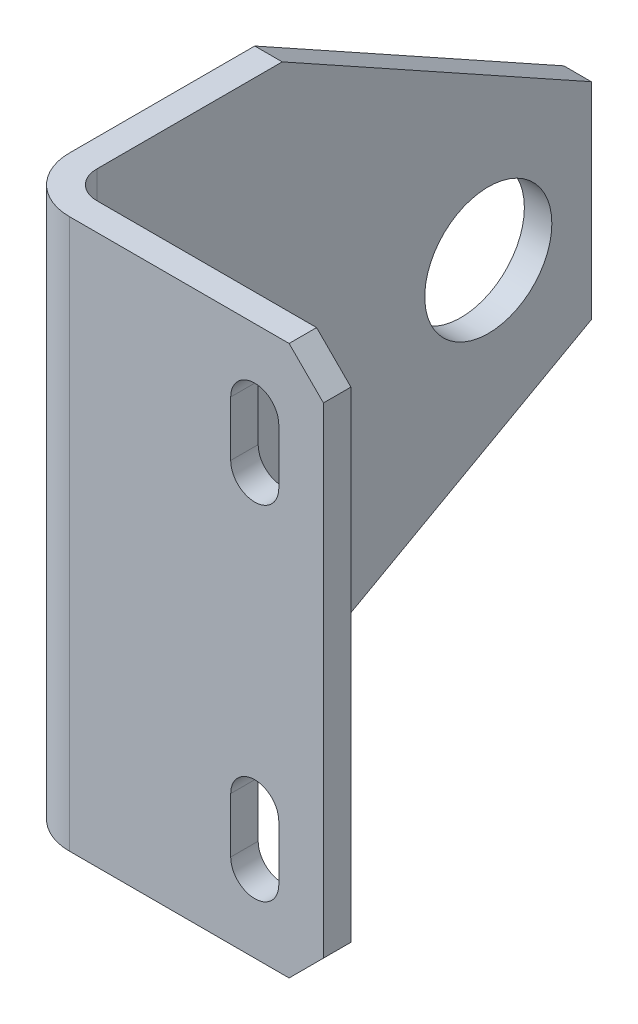
from build123d import *

# Parameters (mm, degrees)
EXTRUDE_1_DEPTH           = 4
SKETCH_2_W                = 4
SKETCH_2_H                = 80
EXTRUDE_2_DEPTH           = 41
CUT_EXTRUDE_1_DEPTH       = 140.749776386
CUT_EXTRUDE_2_DEPTH       = 137.711374801
HOLE_WIZARD_18_5_18_5_1_D = 18.5
CHAMFER_1_SIZE            = 5
CHAMFER_2_SIZE            = 30.886890423
FILLET_1_R                = 4
FILLET_2_R                = 8


with BuildPart() as part:
    # 草图1 → 凸台-拉伸1 (new body)
    with BuildSketch(Plane(origin=(0, 0, 0), x_dir=(0, 0, -1), z_dir=(1, 0, 0))):
        Polygon((-45, 0), (27, 40), (-45, 80), (-80, 80), (-80, 0), align=None)
    extrude(amount=-EXTRUDE_1_DEPTH)

    # 草图2 → 凸台-拉伸2 (add)
    with BuildSketch(Plane(origin=(0, 0, 0), x_dir=(0, 0, -1), z_dir=(1, 0, 0))):
        with Locations((-78, 40)):
            Rectangle(SKETCH_2_W, SKETCH_2_H)
    extrude(amount=EXTRUDE_2_DEPTH)

    # 草图3 → 切除-拉伸1 (cut, through all)
    with BuildSketch(Plane.XY.offset(80)):
        with BuildLine():
            Line((34.5, 61), (34.5, 69))
            ThreePointArc((34.5, 69), (31, 72.5), (27.5, 69))
            Line((27.5, 69), (27.5, 61))
            ThreePointArc((27.5, 61), (31, 57.5), (34.5, 61))
        make_face()
    extrude(amount=-CUT_EXTRUDE_1_DEPTH, mode=Mode.SUBTRACT)

    # 草图4 → 切除-拉伸2 (cut, through all)
    with BuildSketch(Plane(origin=(0, 0, 76), x_dir=(-1, 0, 0), z_dir=(0, 0, -1))):
        with BuildLine():
            Line((-34.5, 19), (-34.5, 11))
            ThreePointArc((-34.5, 11), (-31, 7.5), (-27.5, 11))
            Line((-27.5, 11), (-27.5, 19))
            ThreePointArc((-27.5, 19), (-31, 22.5), (-34.5, 19))
        make_face()
    extrude(amount=-CUT_EXTRUDE_2_DEPTH, mode=Mode.SUBTRACT)

    # Ø18.5 (18.5) 直径孔1 (through all)
    with Locations(Plane(origin=(0, 0, 0), x_dir=(0, 0, -1), z_dir=(1, 0, 0))):
        with Locations((-15, 40)):
            Hole(HOLE_WIZARD_18_5_18_5_1_D / 2)

    # 倒角1
    chamfer_1_edges = [part.edges().sort_by_distance(p)[0] for p in [
        (41, 0, 78),
        (41, 80, 78),
    ]]
    chamfer(chamfer_1_edges, length=CHAMFER_1_SIZE)

    # 倒角2
    chamfer_2_edges = [part.edges().sort_by_distance(p)[0] for p in [
        (-2, 40, -27),
    ]]
    chamfer(chamfer_2_edges, length=CHAMFER_2_SIZE)

    # 圆角1
    fillet_1_edges = [part.edges().sort_by_distance(p)[0] for p in [
        (0, 40, 76),
    ]]
    fillet(fillet_1_edges, radius=FILLET_1_R)

    # 圆角2
    fillet_2_edges = [part.edges().sort_by_distance(p)[0] for p in [
        (-4, 40, 80),
    ]]
    fillet(fillet_2_edges, radius=FILLET_2_R)


solid = part.part
